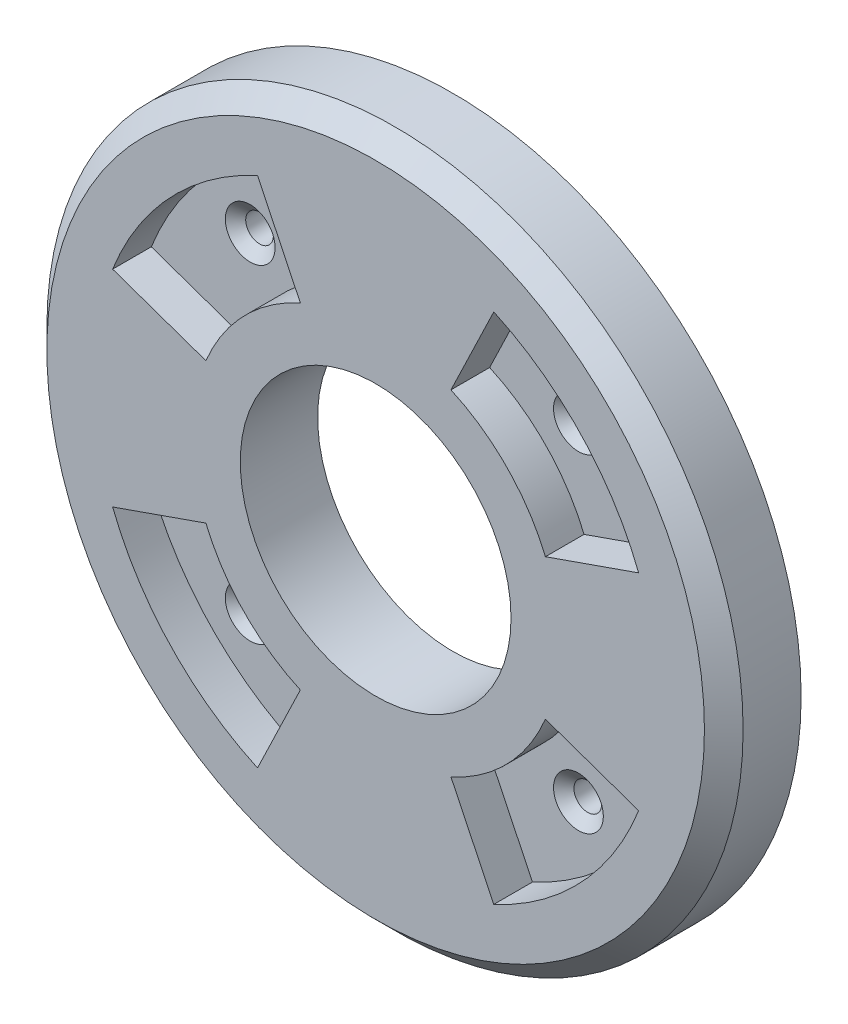
SolidWorks part; units mm, degrees
ref_plane "Front Plane" through (0, 0, 0) normal (0, 0, 1) x (1, 0, 0)
ref_plane "Top Plane" through (0, 0, 0) normal (0, 1, 0) x (1, 0, 0)
ref_plane "Right Plane" through (0, 0, 0) normal (1, 0, 0) x (0, 0, -1)
sketch "Sketch1" plane through (0, 0, 0) normal (0, 0, 1) x (1, 0, 0)
  circle A0 centre (0, 0) radius 90
  circle A1 centre (0, 0) radius 35
  dimension "D1" = 180
  dimension "D2" = 70
extrude "Boss-Extrude1" add sketch "Sketch1" along normal blind 20
sketch "Sketch2" plane through (0, 0, 20) normal (0, 0, 1) x (1, 0, 0)
  line L0 (-138.8179, 0) -> (125.9473, 0) construction
  line L1 (0, 129.8545) -> (0, -159.2728) construction
  line L2 (-19.4683, 43.3271) -> (-30.5424, 66.3272)
  line L3 (-43.8827, 18.1812) -> (-67.9961, 26.6209)
  line L4 (0, 0) -> (-24.7487, 24.7487) construction
  line L5 (43.8827, 18.1812) -> (67.9961, 26.6209)
  line L6 (19.4683, 43.3271) -> (30.5424, 66.3272)
  line L7 (19.4683, -43.3271) -> (30.5424, -66.3272)
  line L8 (43.8827, -18.1812) -> (67.9961, -26.6209)
  line L9 (-43.8827, -18.1812) -> (-67.9961, -26.6209)
  line L10 (-19.4683, -43.3271) -> (-30.5424, -66.3272)
  arc A0 (-30.5424, 66.3272) -> (-67.9961, 26.6209) centre (0, 0) ccw
  arc A1 (43.8827, 18.1812) -> (19.4683, 43.3271) centre (0, 0) ccw
  arc A2 (19.4683, -43.3271) -> (43.8827, -18.1812) centre (0, 0) ccw
  arc A3 (30.5424, 66.3272) -> (67.9961, 26.6209) centre (0, 0) cw
  arc A4 (30.5424, -66.3272) -> (67.9961, -26.6209) centre (0, 0) ccw
  arc A5 (-43.8827, -18.1812) -> (-19.4683, -43.3271) centre (0, 0) ccw
  arc A7 (-30.5424, -66.3272) -> (-67.9961, -26.6209) centre (0, 0) cw
  arc A8 (-19.4683, 43.3271) -> (-43.8827, 18.1812) centre (0, 0) ccw
  dimension "D1" = 45
  dimension "D3" = 95
  dimension "D2" = 45
extrude "Cut-Extrude1" cut sketch "Sketch2" against normal blind 10
chamfer "Chamfer1" distance 5 angle 45 1 edges at (90, 0, 20)
hole_wizard "CSK for 1/4 Flat Head Machine Screw (100)1" positions "Sketch4" profile "Sketch3" countersink size "1/4" standard "Ansi Inch" end condition through all
sketch "Sketch4" plane through (0, 0, 10) normal (0, 0, 1) x (1, 0, 0)
  line L0 (0, 0) -> (0, 142.5226) construction
  line L2 (0, 0) -> (-145.9763, 0) construction
  line L4 (0, 0) -> (-42.4264, 42.4264) construction
  point P0 (-42.4264, 42.4264)
  dimension "D1" = 45
  dimension "D2" = 60
sketch "Sketch3" plane through (-42.4264, 42.4264, 10) normal (1, 0, 0) x (0, -1, 0)
  line L0 (0, 0) -> (0, 10)
  line L1 (0, 10) -> (3.5712, 10)
  line L2 (3.5712, 10) -> (3.5712, 2.4063)
  line L3 (3.5712, 2.4063) -> (6.4389, 0)
  line L5 (6.4389, 0) -> (0, 0)
  line L6 (-3.5712, 2.4063) -> (-6.4389, 0) construction
  line L11 (0, -6.35) -> (0, 107.95) construction
  dimension "通孔孔直径" = 7.1425
  dimension "通孔孔深度" = 10
  dimension "近端锥形沉头孔直径" = 12.8778
  dimension "近端锥形沉头孔角度" = 100
mirror "Mirror1" about plane through (0, 0, 0) normal (1, 0, 0) of "CSK for 1/4 Flat Head Machine Screw (100)1"
mirror "Mirror2" about plane through (0, 0, 0) normal (0, 1, 0) of "CSK for 1/4 Flat Head Machine Screw (100)1", "Mirror1"
